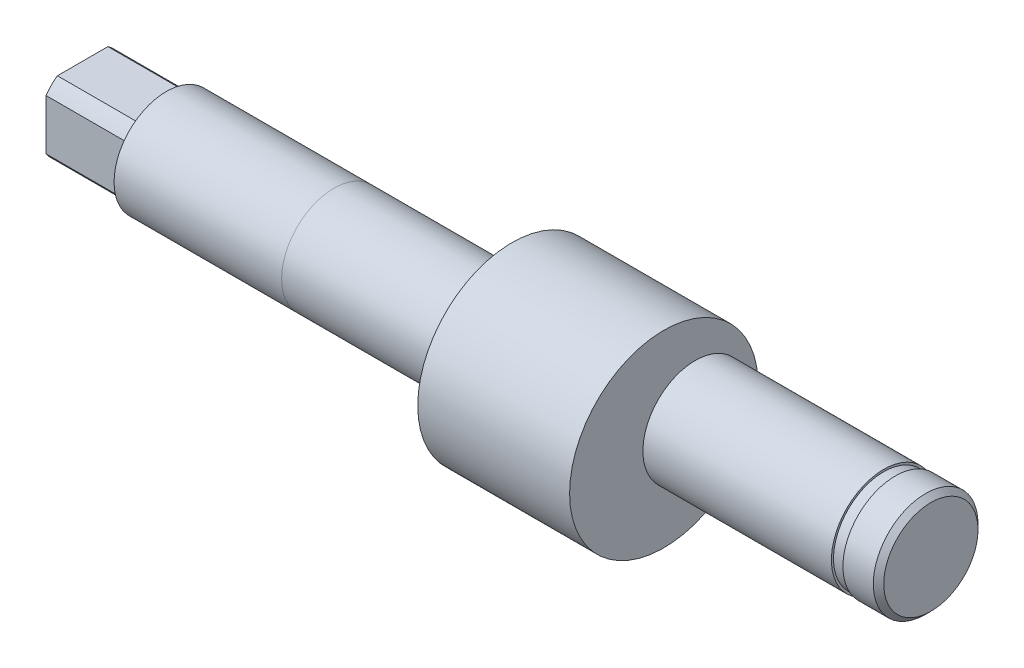
SolidWorks part; units mm, degrees
ref_plane "前视基准面" through (0, 0, 0) normal (0, 0, 1) x (1, 0, 0)
ref_plane "上视基准面" through (0, 0, 0) normal (0, 1, 0) x (1, 0, 0)
ref_plane "右视基准面" through (0, 0, 0) normal (1, 0, 0) x (0, 0, -1)
other "Configuration Table"
sketch "草图2" plane through (0, 0, 0) normal (1, 0, 0) x (0, 0, -1)
  circle A0 centre (0, 0) radius 9
  dimension "D1" = 18
extrude "凸台-拉伸1" add sketch "草图2" along normal blind 14.5
sketch "草图3" plane through (14.5, 0, 0) normal (1, 0, 0) x (0, 0, -1)
  circle A0 centre (3, 0) radius 5
  dimension "D1" = 10
  dimension "D2" = 3
extrude "凸台-拉伸2" add sketch "草图3" along normal blind 18
sketch "草图4" plane through (32.5, 0, 0) normal (1, 0, 0) x (0, 0, -1)
  circle A0 centre (3, 0) radius 4.8
  dimension "D1" = 9.6
extrude "凸台-拉伸3" add sketch "草图4" along normal blind 1.1
sketch "草图5" plane through (33.6, 0, 0) normal (1, 0, 0) x (0, 0, -1)
  circle A0 centre (3, 0) radius 5
  dimension "D1" = 10
extrude "凸台-拉伸4" add sketch "草图5" along normal blind 3.4
chamfer "倒角1" distance 0.5 angle 45 1 edges at (37, 0, -8)
sketch "草图6" plane through (0, 0, 0) normal (-1, 0, 0) x (0, 0, 1)
  circle A0 centre (0, 0) radius 5
  dimension "D1" = 10
extrude "凸台-拉伸5" add sketch "草图6" along normal blind 17
sketch "草图7" plane through (-17, 0, 0) normal (-1, 0, 0) x (0, 0, 1)
  circle A0 centre (0, 0) radius 5
  dimension "D1" = 10
extrude "凸台-拉伸6" add sketch "草图7" along normal blind 16 separate body
cosmetic thread "装饰螺纹线1" parameters "D2"=8.376
sketch "草图8" plane through (-33, 0, 0) normal (-1, 0, 0) x (0, 0, 1)
  line L1 (-2.4109, -3.5) -> (2.4109, -3.5)
  line L2 (-3.5, -2.4109) -> (-3.5, 2.4109)
  line L3 (-2.4109, 3.5) -> (2.4109, 3.5)
  line L4 (3.5, -2.4109) -> (3.5, 2.4109)
  line L5 (0, 3.5) -> (0, -3.5) construction
  line L6 (-3.5, 0) -> (3.5, 0) construction
  arc A0 (-2.4109, 3.5) -> (-3.5, 2.4109) centre (0, 0) ccw
  arc A1 (-3.5, -2.4109) -> (-2.4109, -3.5) centre (0, 0) ccw
  arc A2 (2.4109, -3.5) -> (3.5, -2.4109) centre (0, 0) ccw
  arc A3 (3.5, 2.4109) -> (2.4109, 3.5) centre (0, 0) ccw
  point P0 (0, 0)
  dimension "D1" = 8.5
  dimension "D3" = 3.5
  dimension "D2" = 7
  dimension "D4" = 3.5
extrude "凸台-拉伸7" add sketch "草图8" along normal blind 8
